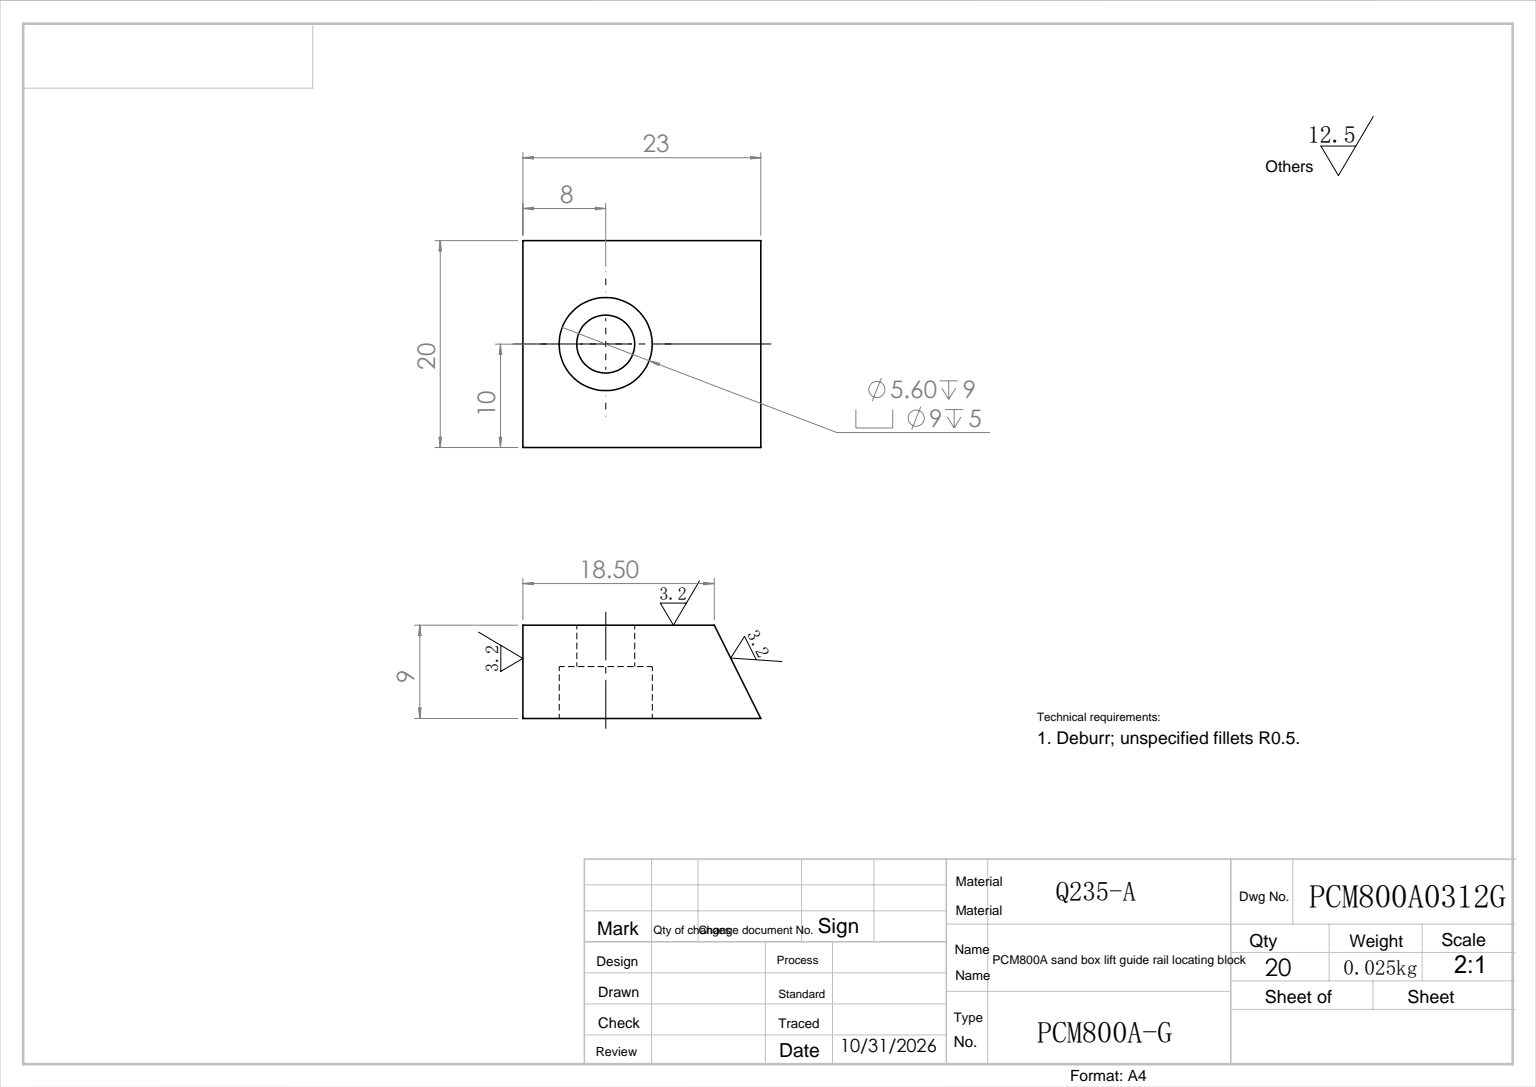
from build123d import *

# Parameters (mm, degrees)
EXTRUDE_1_DEPTH     = 20
SKETCH_2_R          = 4.5
CUT_EXTRUDE_1_DEPTH = 5
SKETCH_3_R          = 2.8
CUT_EXTRUDE_2_DEPTH = 31.886890423


with BuildPart() as part:
    # 草图1 → 拉伸1 (new body)
    with BuildSketch(Plane(origin=(0, 0, 0), x_dir=(1, 0, 0), z_dir=(0, 1, 0))):
        Polygon((0, 0), (18.5, 0), (23, 9), (0, 9), align=None)
    extrude(amount=EXTRUDE_1_DEPTH)

    # 草图2 → 切除-拉伸1 (cut)
    with BuildSketch(Plane(origin=(0, 0, -9), x_dir=(-1, 0, 0), z_dir=(0, 0, -1))):
        with Locations((-8, 10)):
            Circle(SKETCH_2_R)
    extrude(amount=-CUT_EXTRUDE_1_DEPTH, mode=Mode.SUBTRACT)

    # 草图3 → 切除-拉伸2 (cut, through all)
    with BuildSketch(Plane(origin=(0, 0, -4), x_dir=(-1, 0, 0), z_dir=(0, 0, -1))):
        with Locations((-8, 10)):
            Circle(SKETCH_3_R)
    extrude(amount=-CUT_EXTRUDE_2_DEPTH, mode=Mode.SUBTRACT)


solid = part.part
